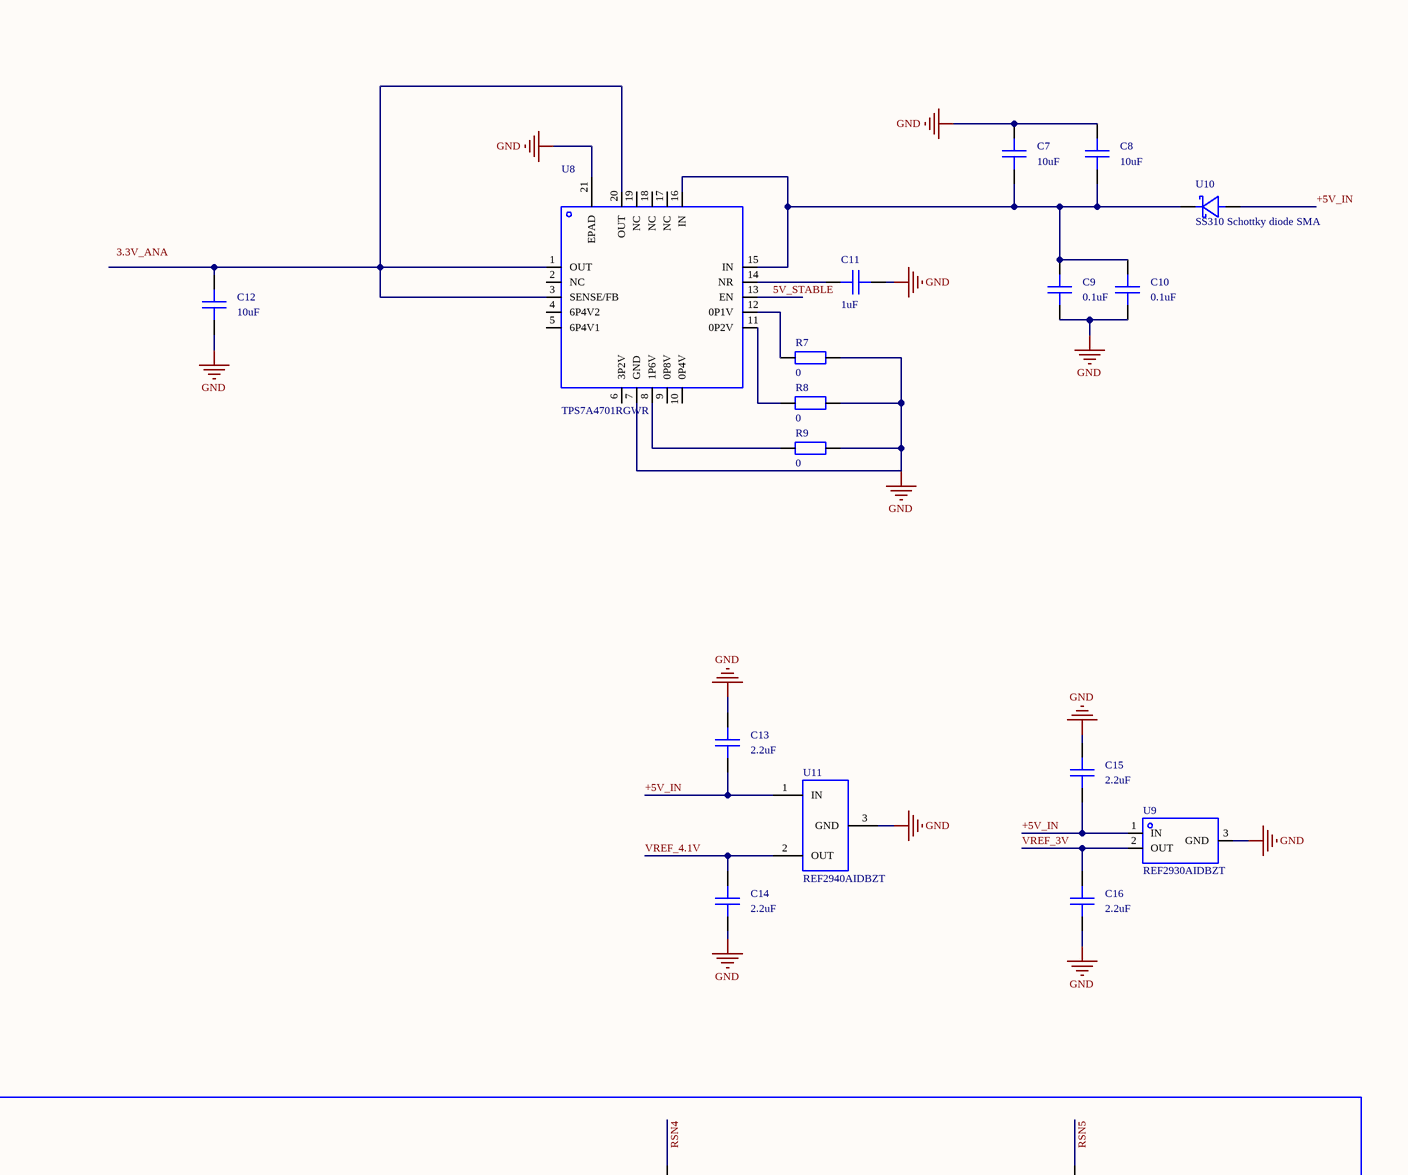
[diagram p0: MISC49874-3.schdoc, top left]
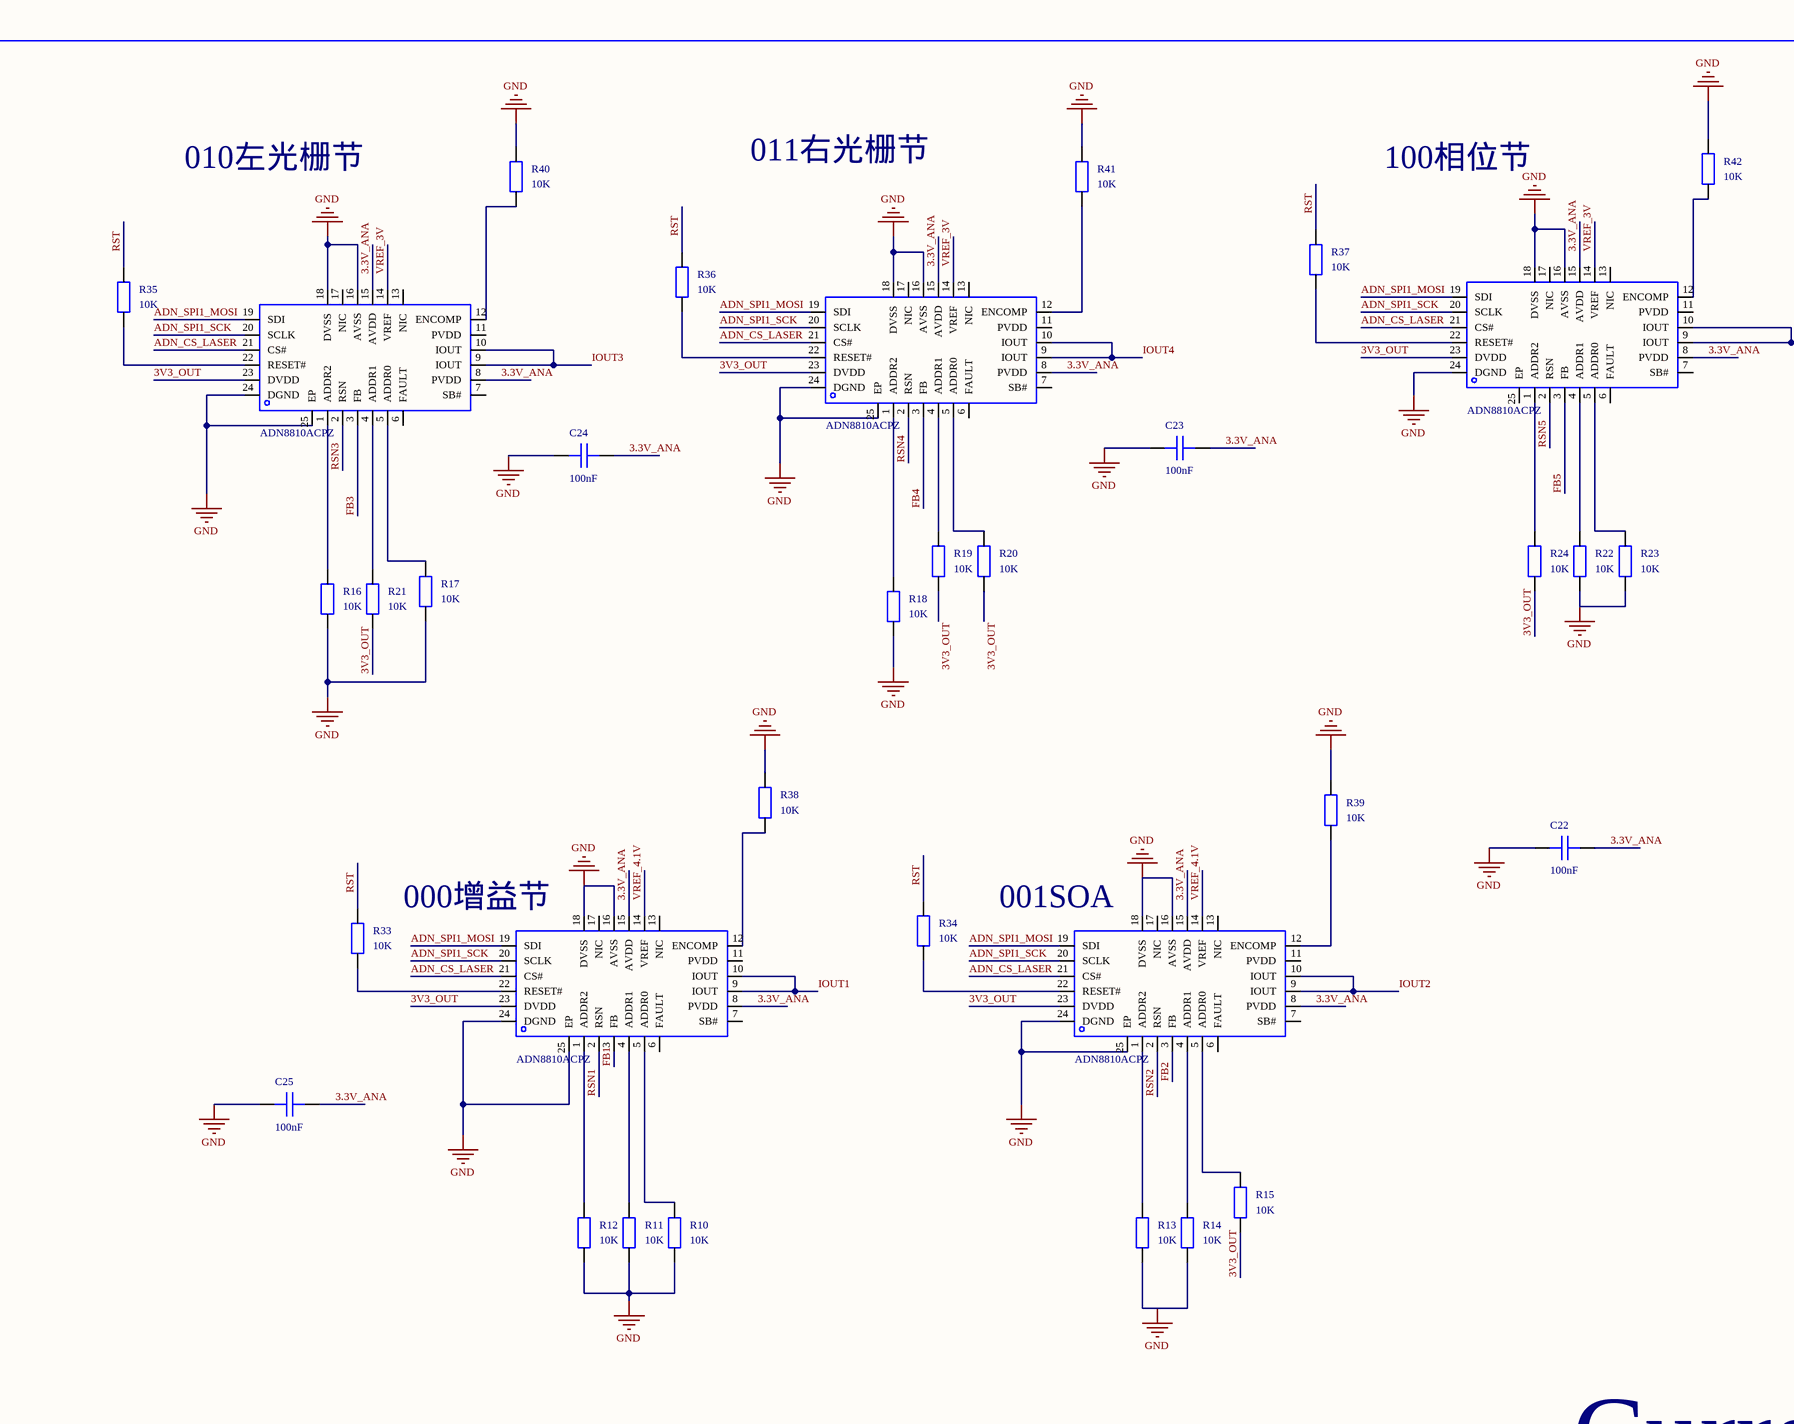
[diagram p1: MISC49874-3.schdoc, top middle]
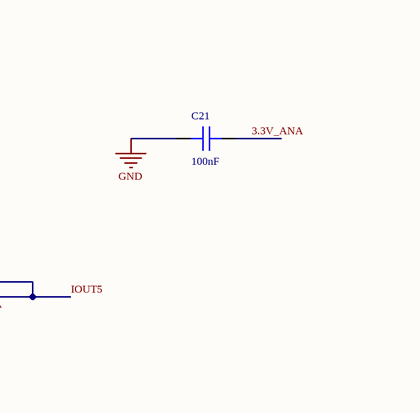
[diagram p2: MISC49874-3.schdoc, top right]
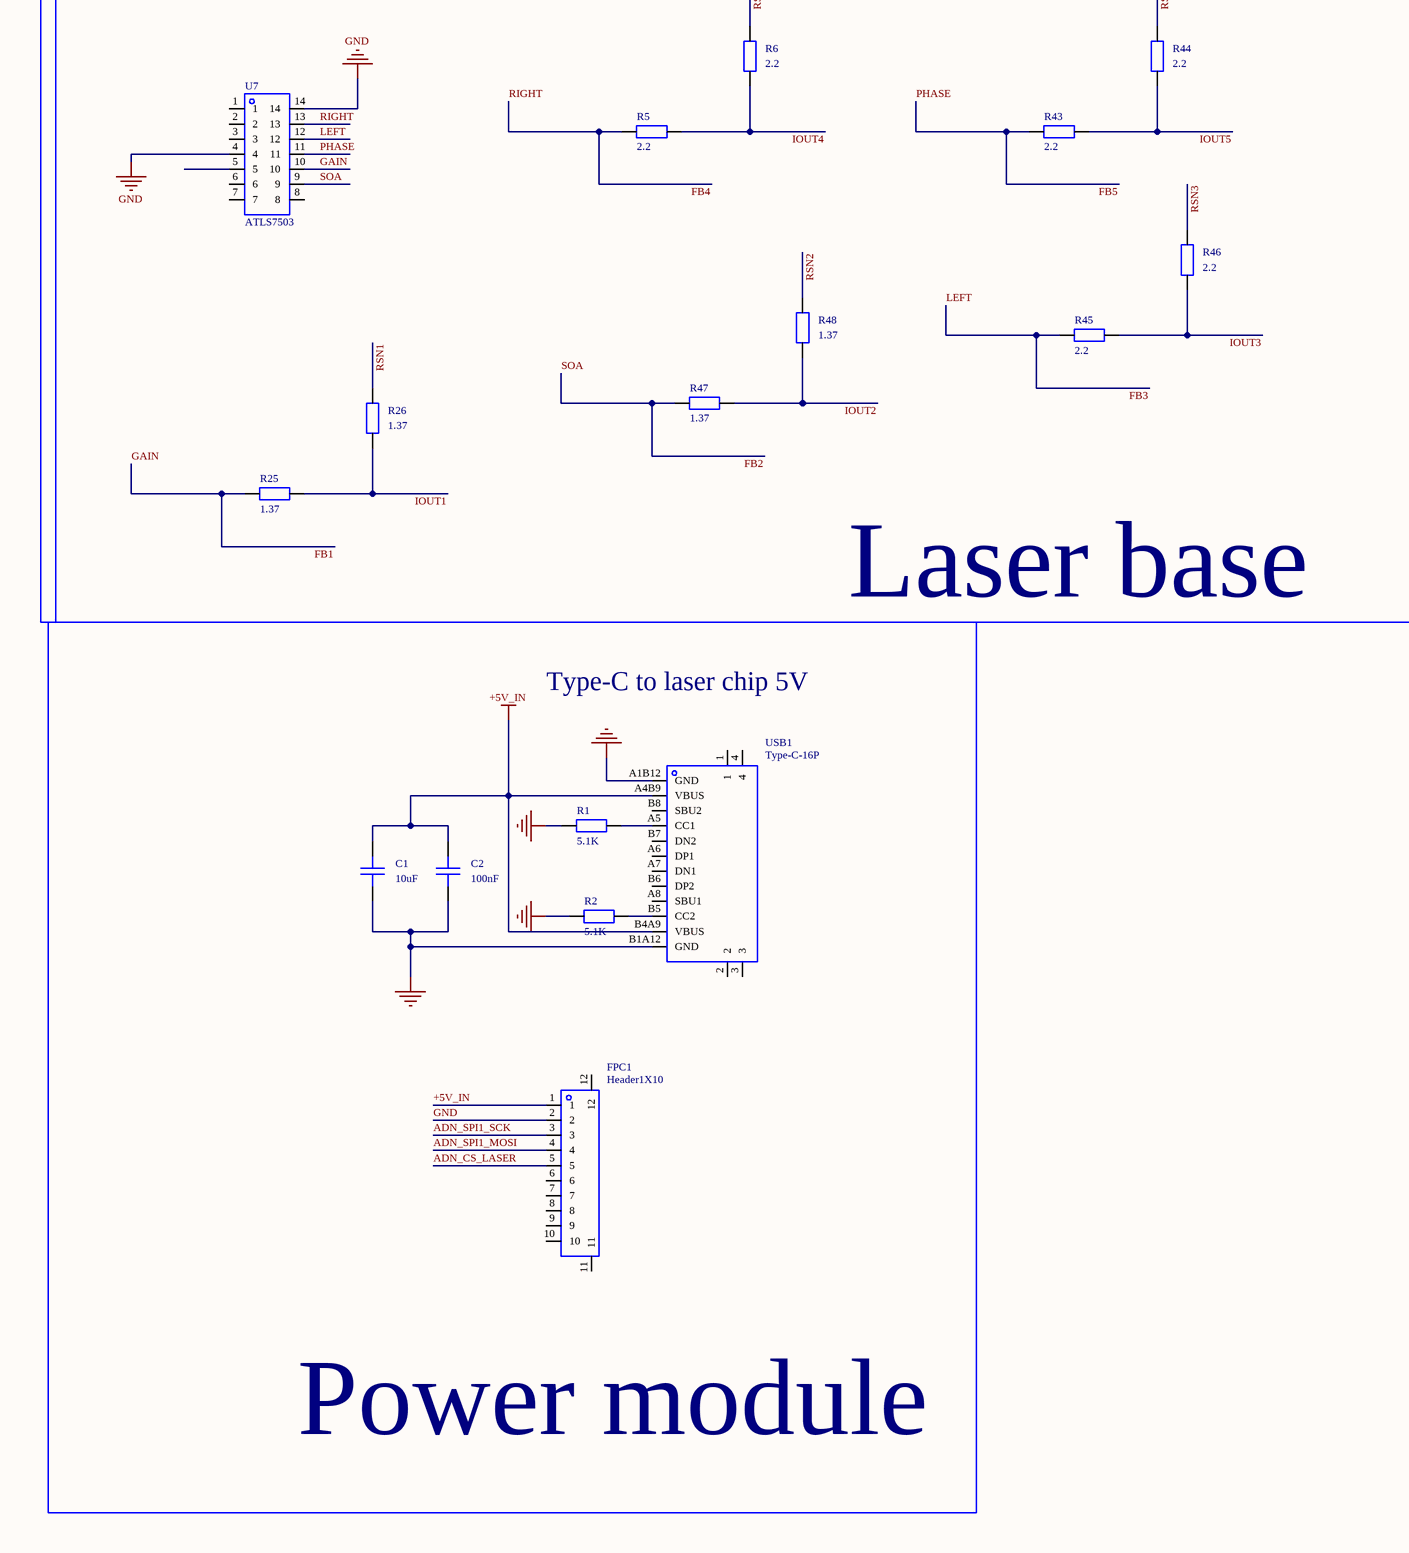
[diagram p3: MISC49874-3.schdoc, bottom left]
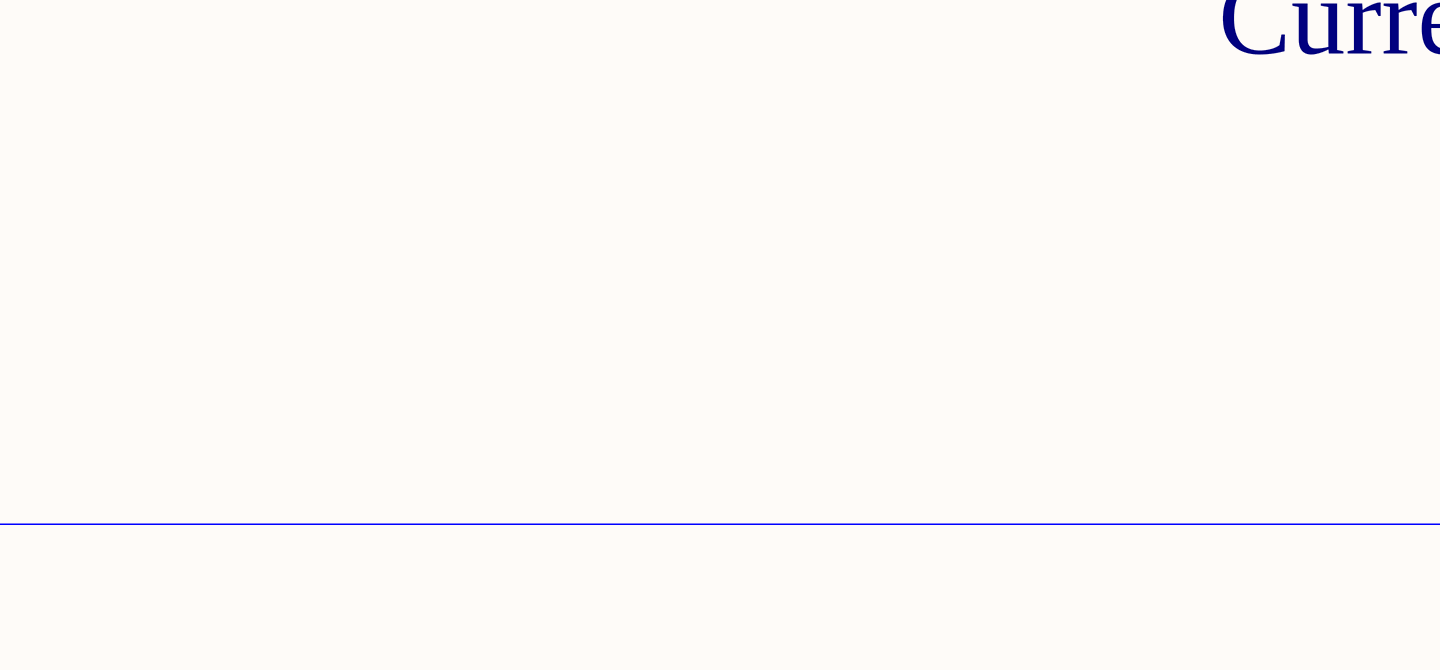
[diagram p4: MISC49874-3.schdoc, bottom middle]
# Altium project MISC49874.PrjPcb
1 sheet, 69 parts. Net scope: global (net labels, ports and power ports of the same name join across sheets).
Board file: MISC49874.pcbdoc

## Sheet MISC49874-3.schdoc
size 635 x 635 mm; @Board Name: MISC49874; @Create Time: 17:30:08; @Page Count: 1; @Page No: 1; @Schematic Name: MISC49874; @Update Time: 17:30:08; Size: A4; Version: V1.0; @Project Name: MISC49874; @Update Date: 2026-03-05; @Create Date: 2026-03-05

### Parts
000增益节  ADN8810ACPZ  [LFCSP-24_L4.0-W4.0-P0.50-BL-EP2.3]
001SOA  ADN8810ACPZ  [LFCSP-24_L4.0-W4.0-P0.50-BL-EP2.3]
010左光栅节  ADN8810ACPZ  [LFCSP-24_L4.0-W4.0-P0.50-BL-EP2.3]
011右光栅节  ADN8810ACPZ  [LFCSP-24_L4.0-W4.0-P0.50-BL-EP2.3]
100相位节  ADN8810ACPZ  [LFCSP-24_L4.0-W4.0-P0.50-BL-EP2.3]
C1  10uF  [C0402]
C2  100nF  [C0402]
C7  10uF  [C0603]
C8  10uF  [C0603]
C9  0.1uF  [C0603]
C10  0.1uF  [C0603]
C11  1uF  [C0603]
C12  10uF  [C0603]
C13  2.2uF  [C0603]
C14  2.2uF  [C0603]
C15  2.2uF  [C0603]
C16  2.2uF  [C0603]
C21  100nF  [C0603]
C22  100nF  [C0603]
C23  100nF  [C0603]
C24  100nF  [C0603]
C25  100nF  [C0603]
FPC1  Header1X10  [FPC-SMD_10P-P1.00_C9900008955]
R1  5.1K  [R0603]
R2  5.1K  [R0603]
R5  2.2  [R0603]
R6  2.2  [R0603]
R7  0  [R0603]
R8  0  [R0603]
R9  0  [R0603]
R10  10K  [R0603]
R11  10K  [R0603]
R12  10K  [R0603]
R13  10K  [R0603]
R14  10K  [R0603]
R15  10K  [R0603]
R16  10K  [R0603]
R17  10K  [R0603]
R18  10K  [R0603]
R19  10K  [R0603]
R20  10K  [R0603]
R21  10K  [R0603]
R22  10K  [R0603]
R23  10K  [R0603]
R24  10K  [R0603]
R25  1.37  [R0603]
R26  1.37  [R0603]
R33  10K  [R0603]
R34  10K  [R0603]
R35  10K  [R0603]
R36  10K  [R0603]
R37  10K  [R0603]
R38  10K  [R0603]
R39  10K  [R0603]
R40  10K  [R0603]
R41  10K  [R0603]
R42  10K  [R0603]
R43  2.2  [R0603]
R44  2.2  [R0603]
R45  2.2  [R0603]
R46  2.2  [R0603]
R47  1.37  [R0603]
R48  1.37  [R0603]
U7  ATLS7503  [HDR-SMD_14P-P1.27-V-F-R2-C7-LS4.8]
U8  TPS7A4701RGWR  [VQFN-20_L5.0-W5.0-P0.65-TL-EP]
U9  REF2930AIDBZT  [SOT-23-3_L2.9-W1.3-P1.90-LS2.4-BR]
U10  SS310 Schottky diode SMA  [SMA_L4.3-W2.6-LS5.1-R-RD]
U11  REF2940AIDBZT  [SOT-23-3_L2.9-W1.3-P1.90-LS2.4-BR]
USB1  Type-C-16P  [USB-C-SMD_GT-USB-7010E]

### Blocks framed on the sheet
Current source module: 000增益节 001SOA 010左光栅节 011右光栅节 100相位节 C7-C16 C21-C25 R7-R24 R33-R42 U8-U11
Laser base: R5 R6 R25 R26 R43-R48 U7

### Nets
+5V_IN: C1.2 C2.2 C13.1 C15.1 FPC1.1 U9.1(IN) U10.1(A) U11.1(IN) USB1.A4B9(VBUS) USB1.B4A9(VBUS)
GND: 000增益节.16(AVSS) 000增益节.18(DVSS) 000增益节.24(DGND) 000增益节.25(EP) 001SOA.16(AVSS) 001SOA.18(DVSS) 001SOA.24(DGND) 001SOA.25(EP) 010左光栅节.16(AVSS) 010左光栅节.18(DVSS) 010左光栅节.24(DGND) 010左光栅节.25(EP) 011右光栅节.16(AVSS) 011右光栅节.18(DVSS) 011右光栅节.24(DGND) 011右光栅节.25(EP) 100相位节.16(AVSS) 100相位节.18(DVSS) 100相位节.24(DGND) C1.1 C2.1 C7.2 C8.2 C9.1 C10.1 C11.1 C12.1 C13.2 C14.1 C15.2 C16.1 C21.2 C22.2 C23.2 C24.2 C25.2 FPC1.2 R1.1 R2.1 R7.2 R8.2 R9.2 R10.1 R11.1 R12.1 R13.1 R14.1 R16.1 R17.1 R18.1 R22.1 R23.1 R38.2 R39.2 R40.2 R41.2 R42.2 U7.4 U7.14 U8.7(GND) U8.21(EPAD) U9.3(GND) U11.3(GND) USB1.A1B12(GND) USB1.B1A12(GND)
3.3V_ANA: 000增益节.8(PVDD) 000增益节.15(AVDD) 001SOA.8(PVDD) 001SOA.15(AVDD) 010左光栅节.8(PVDD) 010左光栅节.15(AVDD) 011右光栅节.8(PVDD) 011右光栅节.15(AVDD) 100相位节.8(PVDD) 100相位节.15(AVDD) C21.1 C22.1 C23.1 C24.1 C25.1
3V3_OUT: 000增益节.23(DVDD) 001SOA.23(DVDD) 010左光栅节.23(DVDD) 011右光栅节.23(DVDD) 100相位节.23(DVDD) R15.1 R19.1 R20.1 R21.1 R24.1
5V_STABLE: U8.13(EN)
ADN_CS_LASER: 000增益节.21(CS#) 001SOA.21(CS#) 010左光栅节.21(CS#) 011右光栅节.21(CS#) 100相位节.21(CS#) FPC1.5
ADN_SPI1_MOSI: 000增益节.19(SDI) 001SOA.19(SDI) 010左光栅节.19(SDI) 011右光栅节.19(SDI) 100相位节.19(SDI) FPC1.4
ADN_SPI1_SCK: 000增益节.20(SCLK) 001SOA.20(SCLK) 010左光栅节.20(SCLK) 011右光栅节.20(SCLK) 100相位节.20(SCLK) FPC1.3
FB1: 000增益节.3(FB) R25.2 U7.10  [also labelled GAIN]
FB2: 001SOA.3(FB) R47.2 U7.9  [also labelled SOA]
FB3: 010左光栅节.3(FB) R45.2 U7.12  [also labelled LEFT]
FB4: 011右光栅节.3(FB) R5.2 U7.13  [also labelled RIGHT]
FB5: 100相位节.3(FB) R43.2 U7.11  [also labelled PHASE]
IOUT1: 000增益节.9(IOUT) 000增益节.10(IOUT) R25.1 R26.2
IOUT2: 001SOA.9(IOUT) 001SOA.10(IOUT) R47.1 R48.2
IOUT3: 010左光栅节.9(IOUT) 010左光栅节.10(IOUT) R45.1 R46.2
IOUT4: 011右光栅节.9(IOUT) 011右光栅节.10(IOUT) R5.1 R6.2
IOUT5: 100相位节.9(IOUT) 100相位节.10(IOUT) R43.1 R44.2
RSN1: 000增益节.2(RSN) R26.1
RSN2: 001SOA.2(RSN) R48.1
RSN3: 010左光栅节.2(RSN) R46.1
RSN4: 011右光栅节.2(RSN) R6.1
RSN5: 100相位节.2(RSN) R44.1
RST: R33.2 R34.2 R35.2 R36.2 R37.2
VREF_3V: 010左光栅节.14(VREF) 011右光栅节.14(VREF) 100相位节.14(VREF) C16.2 U9.2(OUT)
VREF_4.1V: 000增益节.14(VREF) 001SOA.14(VREF) C14.2 U11.2(OUT)
Net000增益节_1: 000增益节.1(ADDR2) R12.2
Net000增益节_4: 000增益节.4(ADDR1) R11.2
Net000增益节_5: 000增益节.5(ADDR0) R10.2
Net000增益节_12: 000增益节.12(ENCOMP) R38.1
Net000增益节_22: 000增益节.22(RESET#) R33.1
Net001SOA_1: 001SOA.1(ADDR2) R13.2
Net001SOA_4: 001SOA.4(ADDR1) R14.2
Net001SOA_5: 001SOA.5(ADDR0) R15.2
Net001SOA_12: 001SOA.12(ENCOMP) R39.1
Net001SOA_22: 001SOA.22(RESET#) R34.1
Net010左光栅节_1: 010左光栅节.1(ADDR2) R16.2
Net010左光栅节_4: 010左光栅节.4(ADDR1) R21.2
Net010左光栅节_5: 010左光栅节.5(ADDR0) R17.2
Net010左光栅节_12: 010左光栅节.12(ENCOMP) R40.1
Net010左光栅节_22: 010左光栅节.22(RESET#) R35.1
Net011右光栅节_1: 011右光栅节.1(ADDR2) R18.2
Net011右光栅节_4: 011右光栅节.4(ADDR1) R19.2
Net011右光栅节_5: 011右光栅节.5(ADDR0) R20.2
Net011右光栅节_12: 011右光栅节.12(ENCOMP) R41.1
Net011右光栅节_22: 011右光栅节.22(RESET#) R36.1
Net100相位节_1: 100相位节.1(ADDR2) R24.2
Net100相位节_4: 100相位节.4(ADDR1) R22.2
Net100相位节_5: 100相位节.5(ADDR0) R23.2
Net100相位节_12: 100相位节.12(ENCOMP) R42.1
Net100相位节_22: 100相位节.22(RESET#) R37.1
NetC7_1: C7.1 C8.1 C9.2 C10.2 U8.15(IN) U8.16(IN) U10.2(K)
NetC11_2: C11.2 U8.14(NR)
NetC12_2: C12.2 U8.1(OUT) U8.3(SENSE/FB) U8.20(OUT)
NetR1_2: R1.2 USB1.A5(CC1)
NetR2_2: R2.2 USB1.B5(CC2)
NetR7_1: R7.1 U8.12(0P1V)
NetR8_1: R8.1 U8.11(0P2V)
NetR9_1: R9.1 U8.8(1P6V)

Not connected (* = marked no-connect by the designer): 000增益节 6(FAULT) 7(SB#) 11(PVDD) 13(NIC) 17(NIC); 001SOA 6(FAULT) 7(SB#) 11(PVDD) 13(NIC) 17(NIC); 010左光栅节 6(FAULT) 7(SB#) 11(PVDD) 13(NIC) 17(NIC); 011右光栅节 6(FAULT) 7(SB#) 11(PVDD) 13(NIC) 17(NIC); 100相位节 6(FAULT) 7(SB#) 11(PVDD) 13(NIC) 17(NIC) 25(EP); FPC1 6 7 8 9 10 11 12; U7 1 2 3 5 6 7 8; U8 2(NC) 4(6P4V2) 5(6P4V1) 6(3P2V) 9(0P8V) 10(0P4V) 17(NC) 18(NC) 19(NC); USB1 1 2 3 4 A6(DP1) A7(DN1) A8(SBU1) B6(DP2) B7(DN2) B8(SBU2)

### Notes on the sheet
- Type-C to laser chip 5V
- Power module
- Labels drawn without touching a wire or pin: 3.3V_ANA
- 2026-03-05
- Schematic
- Board
- Sheet
- P1
- Drawn
- Reviewed
- Revision
- Size
- A4
- page 1 Total 1
- EDA

### Library data of the parts
000增益节 = ADN8810ACPZ: Output current: 300mA;; Manufacturer: ADI(亚德诺); AddInBom: yes; ModelId: fa197dd414874ad2bc21045e91d88c960819f05c4eef4c71ace90d822a990e87; ModelName: LFCSP-24_L4.0-W4.0-H0.8-P0.50; ModelTransform: 157.48,157.48,0,90,0,0,0,0,0; Symbol: ADN8810ACPZ; Device: ADN8810ACPZ; LCSC Part Name: 12位高输出电流源; SupplierPart: C579232; ManufacturerPart: ADN8810ACPZ; Supplier Footprint: LFCSP-24(4x4); JLCPCB Part Class: Extended Part; Datasheet: https://item.szlcsc.com/datasheet/ADN8810ACPZ/607009.html; Supplier: LCSC; ConvertToPcb: yes; FootprintName: LFCSP-24_L4.0-W4.0-P0.50-BL-EP2.3; Type: Current source; Output Current: 300mA; Operating Temperature: -40℃~+85℃
001SOA 010左光栅节 011右光栅节 100相位节 = ADN8810ACPZ: Output current: 300mA;; Manufacturer: ADI(亚德诺); 3D Model: fa197dd414874ad2bc21045e91d88c960819f05c4eef4c71ace90d822a990e87; 3D Model Transform: 157.48,157.48,0,90,0,0,0,0,0; AddInBom: yes; ModelName: LFCSP-24_L4.0-W4.0-H0.8-P0.50; LCSC Part Name: 12位高输出电流源; Supplier Part: C579232; Manufacturer Part: ADN8810ACPZ; Supplier Footprint: LFCSP-24(4x4); JLCPCB Part Class: Extended Part; Datasheet: https://item.szlcsc.com/datasheet/ADN8810ACPZ/607009.html; Supplier: LCSC; Type: Current source; Output Current: 300mA; Operating Temperature: -40℃~+85℃; Symbol: ADN8810ACPZ; Device: ADN8810ACPZ; ConvertToPcb: yes; FootprintName: LFCSP-24_L4.0-W4.0-P0.50-BL-EP2.3
C1 C2 = AC0402KRX7R7BB103: Capacitance: 10nF; accuracy: ±10%; rated voltage: 16V; temperature coefficient: X7R;; Manufacturer: YAGEO(国巨); AddInBom: yes; ModelId: 36a51122f27c49738f86b3bfa98863e00819f05c4eef4c71ace90d822a990e87; ModelName: C0402_L1.0-W0.5-H0.5; ModelTransform: 39.37,19.685,0,0,0,0,0,0,0; Symbol: AC0402KRX7R7BB103; Device: AC0402KRX7R7BB103; LCSC Part Name: 10nF ±10% 16V; ManufacturerPart: AC0402KRX7R7BB103; Supplier Footprint: 0402; JLCPCB Part Class: Extended Part; Datasheet: https://item.szlcsc.com/datasheet/AC0402KRX7R7BB103/773628.html; Supplier: LCSC; ConvertToPcb: yes; FootprintName: C0402; Tolerance: ±10%; Voltage Rating: 16V; Temperature Coefficient: X7R
  C1: Value: 10uF
  C2: Value: 100nF
C7-C10 = CAP_0603: Symbol: Capacitance; ConvertToPcb: yes; ModelId: ac125912035d415993ca9572d50418b10819f05c4eef4c71ace90d822a990e87; ModelName: C0603_L1.6-W0.8-H0.8; ModelTransform: 62.992,31.496,0,0,0,0,0,0,0; Device: CAP_0603; AddInBom: yes; Supplier Footprint: 0603; FootprintName: C0603
  C7 C8: Value: 10uF
  C9 C10: Value: 0.1uF
C11-C16 = CAP_0603: 3D Model: ac125912035d415993ca9572d50418b10819f05c4eef4c71ace90d822a990e87; 3D Model Transform: 62.992,31.496,0,0,0,0,0,0,0; Symbol: Capacitance; ConvertToPcb: yes; ModelName: C0603_L1.6-W0.8-H0.8; Supplier Footprint: 0603; Device: CAP_0603; AddInBom: yes; FootprintName: C0603
  C11: Value: 1uF
  C12: Value: 10uF
  C13-C16: Value: 2.2uF
C21-C25 = CAP_0603: Symbol: Capacitance; 3D Model: ac125912035d415993ca9572d50418b10819f05c4eef4c71ace90d822a990e87; 3D Model Transform: 62.992,31.496,0,0,0,0,0,0,0; ConvertToPcb: yes; ModelName: C0603_L1.6-W0.8-H0.8; Device: CAP_0603; Supplier Footprint: 0603; Value: 100nF; AddInBom: yes; FootprintName: C0603
FPC1 = Header1X10: AddInBom: yes; ModelId: fcc4292dcebf4711a65fd631e94d932e0819f05c4eef4c71ace90d822a990e87; ModelTransform: 583.0697,242.1255,0,0,0,0,0,-56.024,0; Symbol: HEADER1X10; Device: Header1X10; LCSC Part Name: Header1X10; SupplierPart: C9900008955; ManufacturerPart: Header1X10; Supplier Footprint: Header1X10; JLCPCB Part Class: Extended Part; Supplier: LCSC; ConvertToPcb: yes; FootprintName: FPC-SMD_10P-P1.00_C9900008955; ModelName: FPC-SMD_10P-P1.00_C9900008955
R1 R2 = Res_0603: Symbol: Resistor; ConvertToPcb: yes; ModelId: fc143cca1e79419f9cd78b61e9279f080819f05c4eef4c71ace90d822a990e87; ModelTransform: 31.8897,63.7794,0,90,0,0,0,0,0; Value: 5.1K; Device: Res_0603; AddInBom: yes; Supplier Footprint: 0603; FootprintName: R0603; ModelName: R0603
R5 R6 R25 R26 R43-R48 = Res_0603: Symbol: Resistor; 3D Model: fc143cca1e79419f9cd78b61e9279f080819f05c4eef4c71ace90d822a990e87; 3D Model Transform: 31.8897,63.7794,0,90,0,0,0,0,0; ConvertToPcb: yes; Device: Res_0603; Supplier Footprint: 0603; AddInBom: yes; FootprintName: R0603; ModelName: R0603
  R5 R6 R43-R46: Value: 2.2
  R25 R26 R47 R48: Value: 1.37
R7-R24 R33-R42 = Res_0603: 3D Model: fc143cca1e79419f9cd78b61e9279f080819f05c4eef4c71ace90d822a990e87; 3D Model Transform: 31.8897,63.7794,0,90,0,0,0,0,0; Symbol: Resistor; ConvertToPcb: yes; Supplier Footprint: 0603; Device: Res_0603; AddInBom: yes; FootprintName: R0603; ModelName: R0603
  R7-R9: Value: 0
  R10-R24 R33-R42: Value: 10K
U7 = HEADER7X2B: AddInBom: yes; ModelId: 15ced11fe4204b93ba29cc074fdc91ed0819f05c4eef4c71ace90d822a990e87; ModelName: HDR-SMD_14P-P1.27-F-LS-2X7P; ModelTransform: 365.747,188.976,0,0,0,0,0,0,0; Manufacturer Part: ATLS7503; Symbol: HEADER7X2B; Device: HEADER7X2B; LCSC Part Name: HEADER7X2B; SupplierPart: C9900007473; Supplier Footprint: HEADER7X2B; JLCPCB Part Class: Extended Part; Supplier: LCSC; ConvertToPcb: yes; FootprintName: HDR-SMD_14P-P1.27-V-F-R2-C7-LS4.8
U8 = TPS7A4701RGWR: Output type: adjustable; working voltage: 35V; output voltage: 1.4V~34V; output current: 1A; power supply rejection ratio (PSRR): 78dB@(1kHz); output polarity: positive;; Manufacturer: TI(德州仪器); AddInBom: yes; ModelId: eab1241f334749fa99541b9dbcc896380819f05c4eef4c71ace90d822a990e87; ModelName: VQFN-20_L5.0-W5.0-H1.0-P0.65; ModelTransform: 197.6374,197.6374,0,0,0,0,-0.006,0.006,0; Voltage Dropout: 307mV@(1A); Noise: 4uVrms; Number of Outputs: 1; Symbol: TPS7A4701RGWR; Device: TPS7A4701RGWR; LCSC Part Name: 具有使能功能的 1A、36V、低噪声、高 PSRR、低压降稳压器; SupplierPart: C90084; ManufacturerPart: TPS7A4701RGWR; Supplier Footprint: VQFN-20-EP(5x5); JLCPCB Part Class: Extended Part; Supplier: LCSC; ConvertToPcb: yes; FootprintName: VQFN-20_L5.0-W5.0-P0.65-TL-EP; Output Type: Adjustable; Voltage - Supply: 35V; Output Voltage: 1.4V~34V; Output Current: 1A; Power Supply Rejection Ratio (PSRR): 78dB@(1kHz); standby current: -; Features: Overcurrent protection; Operating Temperature: -40℃~+125℃@(Tj); Output Configuration: Positive
U9 = REF2930AIDBZT: Output type: fixed; working voltage: 3.05V~5.5V; output voltage: 3V; output current: 25mA; accuracy: ±2%;; Manufacturer: TI(德州仪器); AddInBom: yes; ModelId: c62791f0466c4ae2a892c056b845b0ca0819f05c4eef4c71ace90d822a990e87; ModelName: SOT-23-3P_L2.9-W1.3-H1.0-LS2.4-P0.95; ModelTransform: 98.425,114.173,0,180,0,0,0.0005,-0.0005,0; Temperature Coefficient: 100ppm/℃; Reference Type: Series; Quiescent Current: 59uA; Symbol: REF2930AIDBZT; Device: REF2930AIDBZT; LCSC Part Name: REF2930AIDBZT; SupplierPart: C2872905; ManufacturerPart: REF2930AIDBZT; Supplier Footprint: SOT-23-3; JLCPCB Part Class: Extended Part; Supplier: LCSC; ConvertToPcb: yes; FootprintName: SOT-23-3_L2.9-W1.3-P1.90-LS2.4-BR; Output Type: Fixed; Voltage - Supply: 3.05V~5.5V; Output Voltage: 3V; Output Current: 25mA; Tolerance: ±2%; Operating Temperature: -40℃~+125℃@(Ta)
U10 = SS310肖特基二极管SMA: AddInBom: yes; ModelId: 6890bb9641474820a71fce2135ca3aaa0819f05c4eef4c71ace90d822a990e87; ModelTransform: 194.8815,98.425,0,0,0,0,0,0,0; Symbol: SS310 Schottky diode SMA; Device: SS310 Schottky diode SMA; LCSC Part Name: SS310肖特基二极管SMA; SupplierPart: C9900014981; ManufacturerPart: SS310肖特基二极管SMA; Supplier Footprint: SS310SMA110V; JLCPCB Part Class: Extended Part; Supplier: LCSC; ConvertToPcb: yes; FootprintName: SMA_L4.3-W2.6-LS5.1-R-RD; ModelName: SMA_L4.3-W2.6-LS5.1-R-RD
U11 = REF2940AIDBZT: Output type: fixed; input voltage: 4.146V~5.5V; output voltage: 4.096V; output current: 25mA; accuracy: ±2%;; Manufacturer: TI(德州仪器); AddInBom: yes; ModelId: c62791f0466c4ae2a892c056b845b0ca0819f05c4eef4c71ace90d822a990e87; ModelName: SOT-23-3P_L2.9-W1.3-H1.0-LS2.4-P0.95; ModelTransform: 98.425,114.173,0,180,0,0,0.0005,-0.0005,0; Temperature Coefficient: 100ppm/℃; Reference Type: Series; Supply Current: 59uA; Noise - 1/10Hz to 10Hz: 45uVp-p; Noise - 10Hz to 10kHz: 128uVrms; Symbol: REF2940AIDBZT; Device: REF2940AIDBZT; LCSC Part Name: REF2940AIDBZT; SupplierPart: C111864; ManufacturerPart: REF2940AIDBZT; Supplier Footprint: SOT-23; JLCPCB Part Class: Extended Part; Supplier: LCSC; ConvertToPcb: yes; FootprintName: SOT-23-3_L2.9-W1.3-P1.90-LS2.4-BR; Output Type: Fixed; Input Voltage: 4.146V~5.5V; Output Voltage: 4.096V; Output Current: 25mA; Tolerance: ±2%; Operating Temperature: -40℃~+125℃@(Ta)
USB1 = Type-C-16P: AddInBom: yes; ModelId: 5afd3849e9c642128e878b8e27a760ba0819f05c4eef4c71ace90d822a990e87; ModelTransform: 351.9678,304.33,0,0,0,0,0,-43.307,-35.433; Symbol: TYPE-C-16P; Device: Type-C-16P; LCSC Part Name: Type-C-16P; SupplierPart: C9900216560; ManufacturerPart: Type-C-16P; Supplier Footprint: SMD; JLCPCB Part Class: Extended Part; Supplier: LCSC; ConvertToPcb: yes; FootprintName: USB-C-SMD_GT-USB-7010E; ModelName: USB-C-SMD_GT-USB-7010E